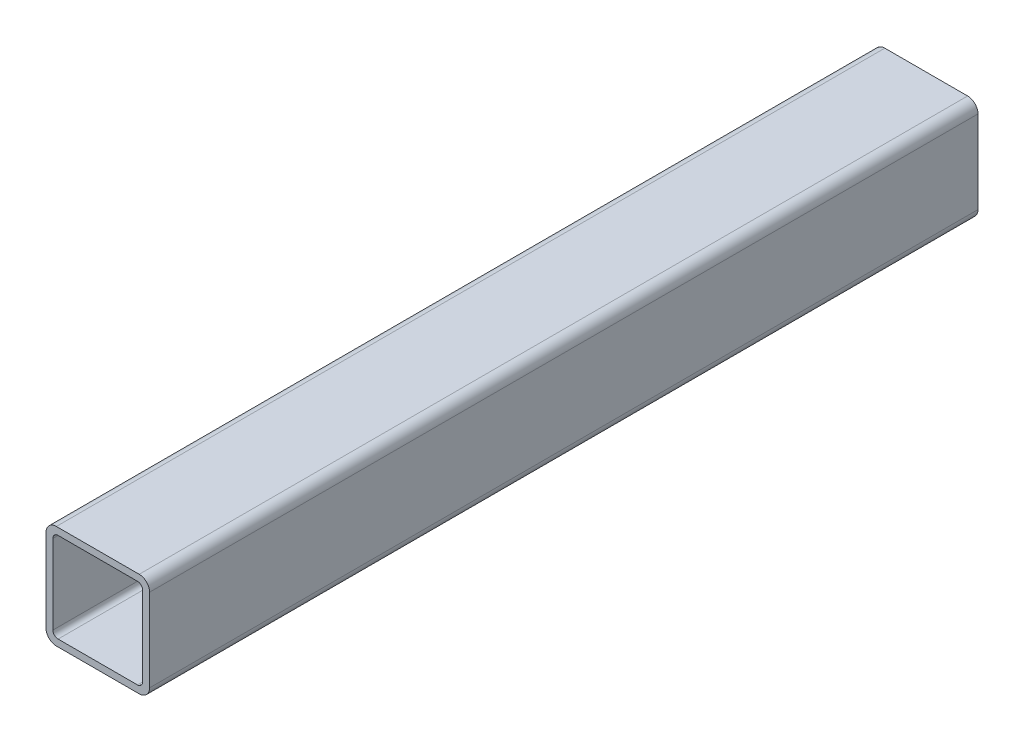
from build123d import *

# Parameters (mm, degrees)
SKETCH1_W           = 60
SKETCH1_H           = 60
SKETCH1_W_2         = 52
SKETCH1_H_2         = 52
BOSS_EXTRUDE1_DEPTH = 240
FILLET1_R           = 6
FILLET2_R           = 3


with BuildPart() as part:
    # Sketch1 → Boss-Extrude1 (new, symmetric)
    with BuildSketch(Plane.XY):
        Rectangle(SKETCH1_W, SKETCH1_H)
        Rectangle(SKETCH1_W_2, SKETCH1_H_2, mode=Mode.SUBTRACT)
    extrude(amount=BOSS_EXTRUDE1_DEPTH, both=True)

    # Fillet1
    fillet1_edges = [part.edges().sort_by_distance(p)[0] for p in [
        (30, -30, 0),
        (-30, -30, 0),
        (-30, 30, 0),
        (30, 30, 0),
    ]]
    fillet(fillet1_edges, radius=FILLET1_R)

    # Fillet2
    fillet2_edges = [part.edges().sort_by_distance(p)[0] for p in [
        (26, -26, 0),
        (26, 26, 0),
        (-26, 26, 0),
        (-26, -26, 0),
    ]]
    fillet(fillet2_edges, radius=FILLET2_R)


solid = part.part
